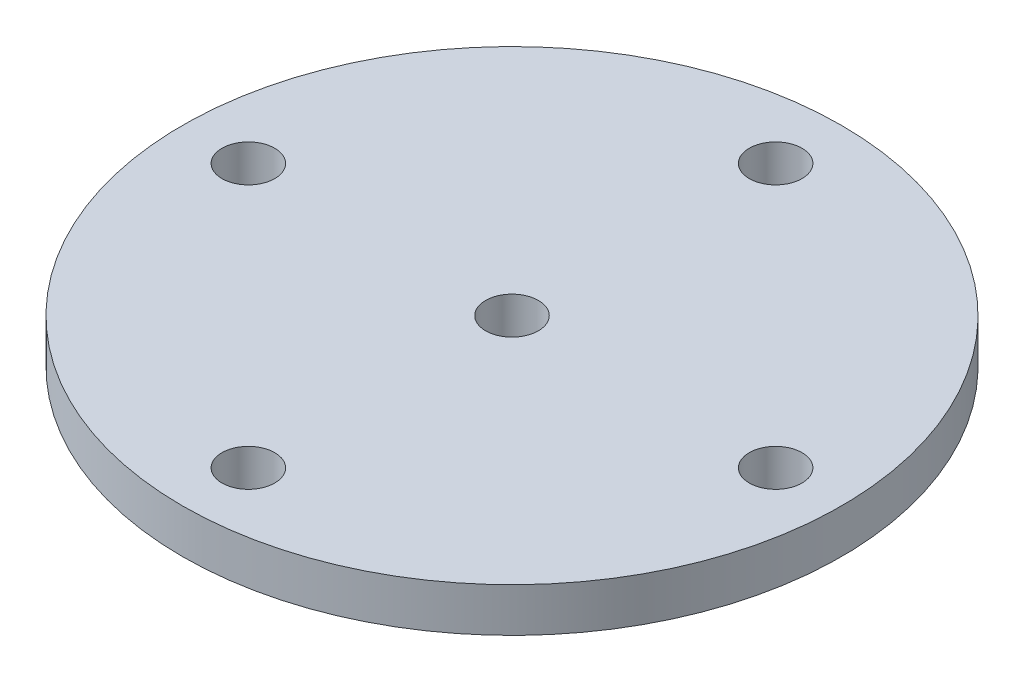
SolidWorks part; units mm, degrees
material "普通碳钢"
ref_plane "Front Plane" through (0, 0, 0) normal (0, 0, 1) x (1, 0, 0)
ref_plane "Top Plane" through (0, 0, 0) normal (0, 1, 0) x (1, 0, 0)
ref_plane "Right Plane" through (0, 0, 0) normal (1, 0, 0) x (0, 0, -1)
other "Configuration Table"
sketch "Sketch1" plane through (0, 0, 0) normal (0, 1, 0) x (1, 0, 0)
  circle A0 centre (0, 0) radius 75
  dimension "D1" = 150
extrude "Boss-Extrude1" add sketch "Sketch1" along normal blind 10
sketch "Sketch2" plane through (0, 10, 0) normal (0, 1, 0) x (1, 0, 0)
  circle A0 centre (0, 60) radius 6
  circle A1 centre (0, 0) radius 6
  circle A2 centre (0, -60) radius 6
  circle A3 centre (-60, 0) radius 6
  circle A4 centre (60, 0) radius 6
  dimension "D1" = 12
  dimension "D3" = 60
  dimension "D4" = 12
  dimension "D5" = 12
  dimension "D2" = 60
  dimension "D6" = 60
  dimension "D7" = 60
extrude "Cut-Extrude1" cut sketch "Sketch2" against normal through all
